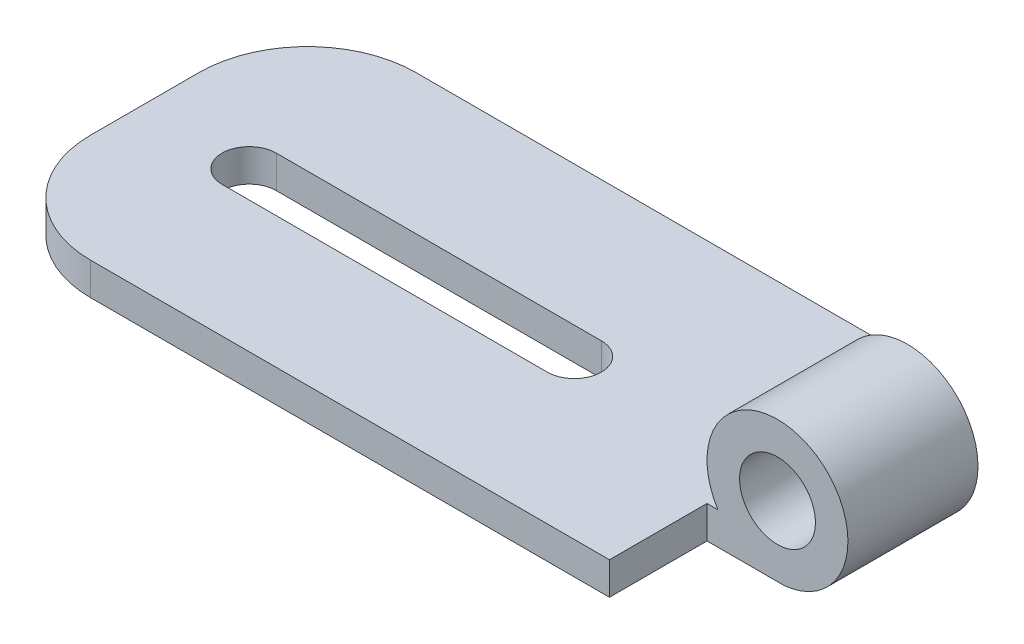
from build123d import *

# Parameters (mm, degrees)
SKETCH_1_R          = 3.5
EXTRUDE_1_DEPTH     = 30
FILLET_1_R          = 10
CUT_EXTRUDE_1_DEPTH = 30
SKETCH_3_W          = 18.572765592
SKETCH_3_H          = 9
SKETCH_3_W_2        = 28.522519482
CUT_EXTRUDE_2_DEPTH = 15


with BuildPart() as part:
    # 草图1 → 凸台-拉伸1 (new body)
    with BuildSketch(Plane.XY):
        with BuildLine():
            Line((-32.5, 1.5), (26.367564687, 1.5))
            ThreePointArc((26.367564687, 1.5), (34.720903057, 10.807641922), (32.5, -1.5))
            Line((32.5, -1.5), (-32.5, -1.5))
            Line((-32.5, -1.5), (-32.5, 1.5))
        make_face()
        with Locations((31.86456148, 4.96886527)):
            Circle(SKETCH_1_R, mode=Mode.SUBTRACT)
    extrude(amount=EXTRUDE_1_DEPTH)

    # 圆角1
    fillet_1_edges = [part.edges().sort_by_distance(p)[0] for p in [
        (-32.5, 0, 30),
        (-32.5, 0, 0),
    ]]
    fillet(fillet_1_edges, radius=FILLET_1_R)

    # 草图2 → 切除-拉伸1 (cut)
    with BuildSketch(Plane(origin=(0, 1.5, 0), x_dir=(1, 0, 0), z_dir=(0, 1, 0))):
        with BuildLine():
            Line((-22.5, -12.87764733), (7.5, -12.87764733))
            ThreePointArc((7.5, -12.87764733), (10, -15.37764733), (7.5, -17.87764733))
            Line((7.5, -17.87764733), (-22.5, -17.87764733))
            ThreePointArc((-22.5, -17.87764733), (-25, -15.37764733), (-22.5, -12.87764733))
        make_face()
    extrude(amount=-CUT_EXTRUDE_1_DEPTH, mode=Mode.SUBTRACT)

    # 草图3 → 切除-拉伸2 (cut, symmetric)
    with BuildSketch(Plane(origin=(0, 1.5, 0), x_dir=(1, 0, 0), z_dir=(0, 1, 0))):
        with Locations((34.650944276, -25.5)):
            Rectangle(SKETCH_3_W, SKETCH_3_H)
        with Locations((39.625821221, -4.5)):
            Rectangle(SKETCH_3_W_2, SKETCH_3_H)
    extrude(amount=CUT_EXTRUDE_2_DEPTH, both=True, mode=Mode.SUBTRACT)


solid = part.part
